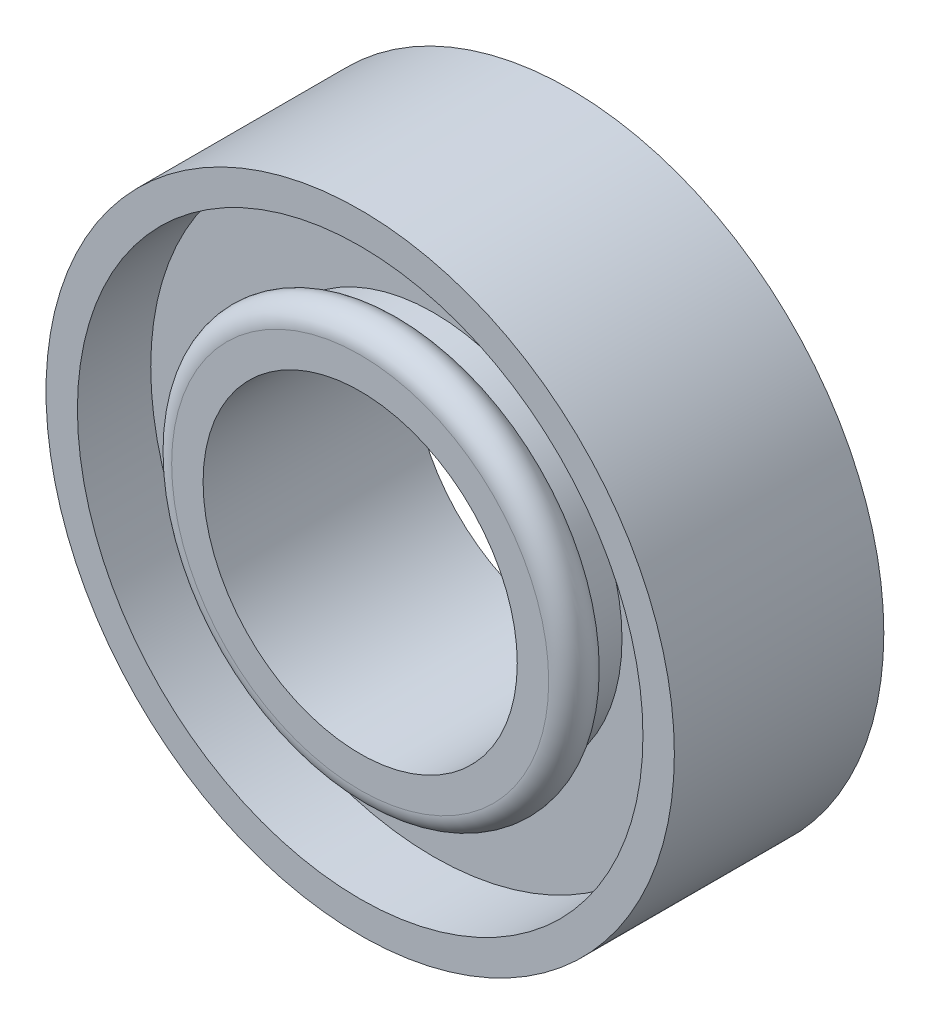
SolidWorks part; units mm, degrees
ref_plane "前视基准面" through (0, 0, 0) normal (0, 0, 1) x (1, 0, 0)
ref_plane "上视基准面" through (0, 0, 0) normal (0, 1, 0) x (1, 0, 0)
ref_plane "右视基准面" through (0, 0, 0) normal (1, 0, 0) x (0, 0, -1)
sketch "草图1" plane through (0, 0, 0) normal (1, 0, 0) x (0, 0, -1)
  line L0 (0, 15) -> (0, 7.5)
  line L1 (0, 7.5) -> (5, 7.5)
  line L2 (5, 7.5) -> (5, 9)
  line L3 (0, 15) -> (5, 15)
  line L4 (5, 15) -> (5, 13.5)
  line L5 (5, 13.5) -> (1.5, 13.5)
  line L6 (3, 9) -> (1.5, 9)
  line L7 (1.5, 9) -> (1.5, 13.5)
  line L8 (-4.2174, 0) -> (8.8764, 0) construction
  arc A0 (3, 9) -> (5, 9) centre (4, 9) cw
  dimension "D8" = 1
  dimension "D1" = 7.5
  dimension "D2" = 15
  dimension "D3" = 5
  dimension "D4" = 1.5
  dimension "D5" = 1.5
  dimension "D7" = 1.5
  dimension "D9" = 5
revolve "旋转2" add sketch "草图1" angle 360 about L8
mirror "镜向2" about plane through (0, 15, 0) normal (0, 0, -1) of "旋转2"
